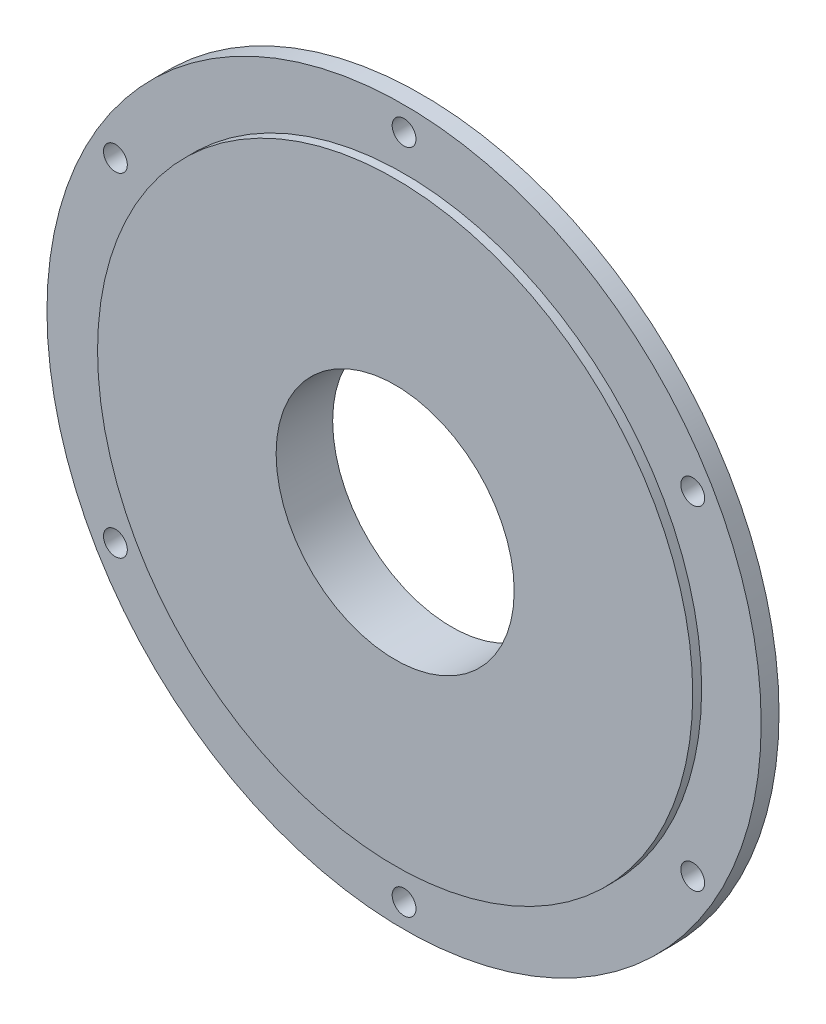
SolidWorks part; units mm, degrees
material "HT200"
ref_plane "Front Plane" through (0, 0, 0) normal (0, 0, 1) x (1, 0, 0)
ref_plane "Top Plane" through (0, 0, 0) normal (0, 1, 0) x (1, 0, 0)
ref_plane "Right Plane" through (0, 0, 0) normal (1, 0, 0) x (0, 0, -1)
other "Configuration Table"
sketch "Sketch1" plane through (0, 0, 0) normal (0, 1, 0) x (1, 0, 0)
  line L0 (0, 4.9569) -> (0, 0) construction
  line L1 (20, 9.5) -> (20, 0)
  line L2 (50, 1.5) -> (60, 1.5)
  line L3 (60, 1.5) -> (60, 4.5)
  line L4 (60, 4.5) -> (23, 4.5)
  line L5 (23, 4.5) -> (23, 9.5)
  line L6 (23, 9.5) -> (20, 9.5)
  line L7 (50, 1.5) -> (50, 0)
  line L8 (50, 0) -> (20, 0)
  line L10 (-2.237, 0) -> (1.808, 0) construction
  point P4 (50, 0.75)
  dimension "D1" = 3
  dimension "D2" = 1.5
  dimension "D3" = 60
  dimension "D4" = 50
  dimension "D5" = 20
  dimension "D6" = 3
  dimension "D7" = 5
revolve "Revolve1" add sketch "Sketch1" angle 360 about L0
sketch "Sketch2" plane through (0, 0, -4.5) normal (0, 0, -1) x (-1, 0, 0)
  circle A0 centre (0, 0) radius 56 construction
  circle A1 centre (0, 56) radius 2
  circle A2 centre (48.4974, 28) radius 2
  circle A3 centre (48.4974, -28) radius 2
  circle A4 centre (0, -56) radius 2
  circle A5 centre (-48.4974, -28) radius 2
  circle A6 centre (-48.4974, 28) radius 2
  point P17 (0, 0)
  dimension "D1" = 112
  dimension "D2" = 4
  dimension "D3" = 6
extrude "Cut-Extrude1" cut sketch "Sketch2" against normal blind 10 contours A1 | A6 | A5 | A4 | A3 | A2
